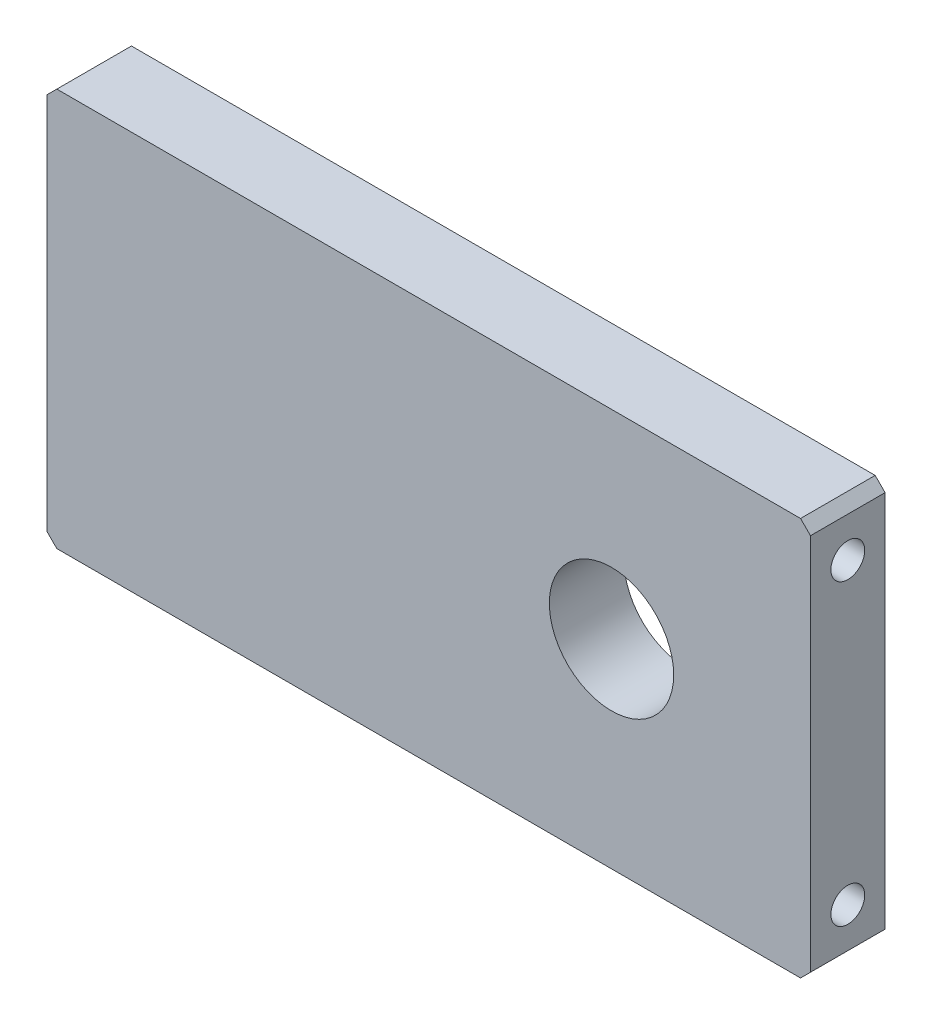
from build123d import *

# Parameters (mm, degrees)
SKETCH_1_W                  = 153.5
SKETCH_1_H                  = 80
EXTRUDE_1_DEPTH             = 7.5
HOLE_WIZARD_25_0_25_1_D     = 25
HOLE_WIZARD_M8_1_AT_2_COUNT = 2
HOLE_WIZARD_M8_1_AT_2_PITCH = 60
CHAMFER_1_SIZE              = 2


with BuildPart() as part:
    # 草图1 → 凸台-拉伸1 (new, symmetric)
    with BuildSketch(Plane.XY):
        Rectangle(SKETCH_1_W, SKETCH_1_H)
    extrude(amount=EXTRUDE_1_DEPTH, both=True)

    # Ø25.0 (25) 直径孔1 (through all)
    with Locations(Plane.XY.offset(7.5)):
        with Locations((36.75, 0)):
            Hole(HOLE_WIZARD_25_0_25_1_D / 2)

    # 草图4 → M8 螺纹孔1 (revolve, cut)
    with BuildSketch(Plane(origin=(76.75, 30, 0), x_dir=(0, 0, -1), z_dir=(0, 1, 0))):
        Polygon((0, 0), (0, 21.792926105), (3.4, 19.75), (3.4, 0), align=None)
    hole_wizard_m8_1 = revolve(axis=Axis((83.1, 30, 0), (-1, 0, 0)), mode=Mode.SUBTRACT)

    # M8 螺纹孔1 at 2: M8 螺纹孔1 ×2
    with Locations(*[(0, -i * HOLE_WIZARD_M8_1_AT_2_PITCH, 0) for i in range(1, HOLE_WIZARD_M8_1_AT_2_COUNT)]):
        add(hole_wizard_m8_1, mode=Mode.SUBTRACT)

    # 镜向1: M8 螺纹孔1 across plane
    add(hole_wizard_m8_1.mirror(Plane(origin=(0, 0, 0), x_dir=(0, 0, 1), z_dir=(1, 0, 0))), mode=Mode.SUBTRACT)

    # 镜向1 copy 1 sketch → 镜向1 copy 1 (revolve, cut)
    with BuildSketch(Plane(origin=(-76.75, -30, 0), x_dir=(0, 0, -1), z_dir=(0, 1, 0))):
        Polygon((0, 0), (0, -21.792926105), (3.4, -19.75), (3.4, 0), align=None)
    revolve(axis=Axis((-83.1, -30, 0), (-1, 0, 0)), mode=Mode.SUBTRACT)

    # 倒角1
    chamfer_1_edges = [part.edges().sort_by_distance(p)[0] for p in [
        (76.75, -40, 0),
        (-76.75, -40, 0),
        (-76.75, 40, 0),
        (76.75, 40, 0),
    ]]
    chamfer(chamfer_1_edges, length=CHAMFER_1_SIZE)


solid = part.part
